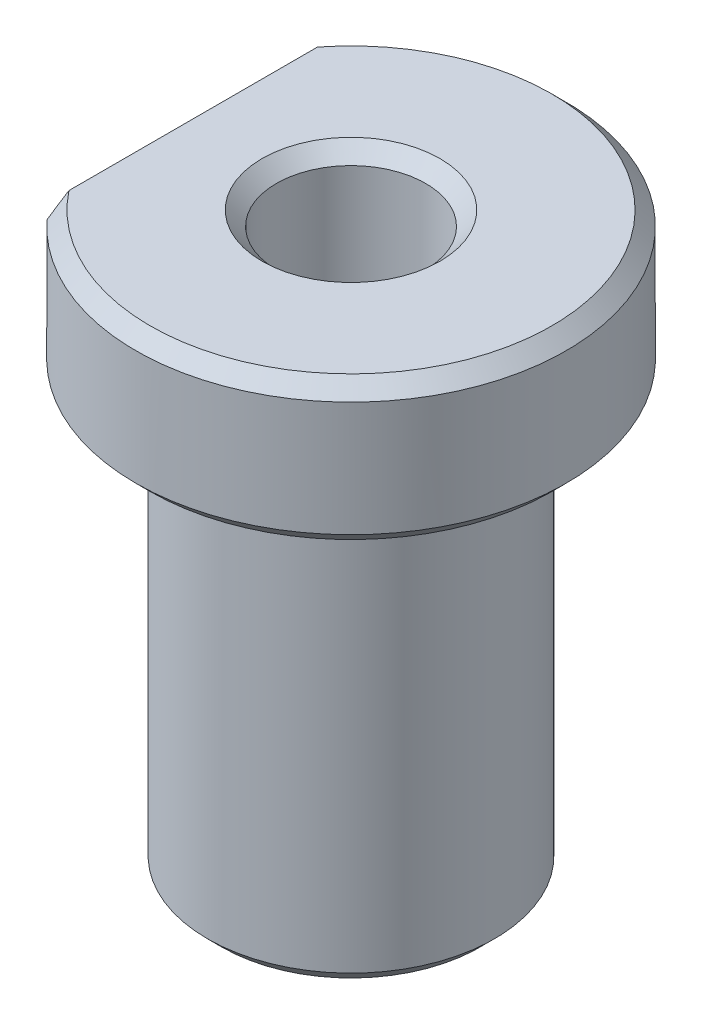
SolidWorks part; units mm, degrees
material "S45C"
ref_plane "Front Plane" through (0, 0, 0) normal (0, 0, 1) x (1, 0, 0)
ref_plane "Top Plane" through (0, 0, 0) normal (0, 1, 0) x (1, 0, 0)
ref_plane "Right Plane" through (0, 0, 0) normal (1, 0, 0) x (0, 0, -1)
sketch "Sketch1" plane through (0, 0, 0) normal (0, 1, 0) x (1, 0, 0)
  circle A0 centre (0, 0) radius 5
  circle A1 centre (0, 0) radius 2.6
  dimension "D1" = 5.2
  dimension "D2" = 10
extrude "Boss-Extrude1" add sketch "Sketch1" along normal blind 15
sketch "Sketch2" plane through (0, 15, 0) normal (0, 1, 0) x (1, 0, 0)
  circle A0 centre (0, 0) radius 2.6 construction
  circle A1 centre (0, 0) radius 2.6
  circle A2 centre (0, 0) radius 7.5
  dimension "D1" = 15
extrude "Boss-Extrude2" add sketch "Sketch2" along normal blind 5
chamfer "Chamfer1" distance 0.5 angle 45 4 edges at (0, 15, 7.5) (0, 20, 7.5) (0, 0, 5) (0, 20, 2.6)
sketch "Sketch3" plane through (0, 0, 0) normal (0, 0, 1) x (1, 0, 0)
  line L0 (-7.5, 19.5) -> (-7.5, 15.5) construction
  line L1 (-10.5, 23) -> (-5.5, 23)
  line L2 (-10.5, 23) -> (-10.5, 18)
  line L3 (-10.5, 18) -> (-5.5, 18)
  line L4 (-5.5, 23) -> (-5.5, 18)
  line L5 (-7, 15) -> (7, 15) construction
  dimension "D1" = 2
  dimension "D2" = 3
  dimension "D3" = 5
  dimension "D4" = 5
extrude "Cut-Extrude1" cut sketch "Sketch3" against normal mid plane 50
